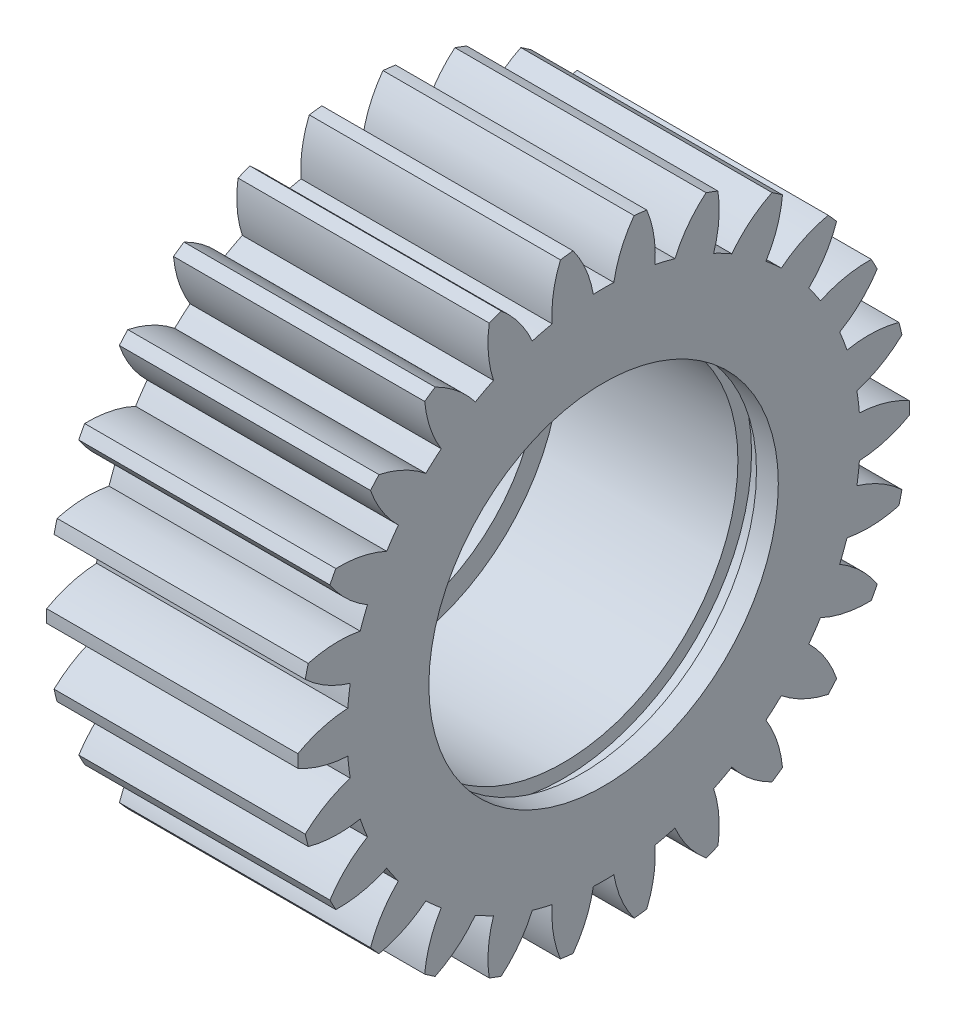
SolidWorks part; units mm, degrees
ref_plane "前视基准面" through (0, 0, 0) normal (0, 0, 1) x (1, 0, 0)
ref_plane "上视基准面" through (0, 0, 0) normal (0, 1, 0) x (1, 0, 0)
ref_plane "右视基准面" through (0, 0, 0) normal (1, 0, 0) x (0, 0, -1)
ref_plane "基准面4" through (0, 0, 0) normal (0, 0, -1) x (-1, 0, 0)
sketch "草图1" plane through (0, 0, 0) normal (0, 0, -1) x (-1, 0, 0)
  line L0 (-20, 28) -> (-20, 0)
  line L1 (-20, 0) -> (3, 0)
  line L2 (3, 0) -> (3, 28)
  line L3 (3, 28) -> (-20, 28)
  line L4 (-20, 0) -> (3, 0) construction
revolve "旋转1" add sketch "草图1" angle 360 about L4
sketch "草图2" plane through (-3, 0, 0) normal (-1, 0, 0) x (0, 0, 1)
  arc A0 (27.0412, 7.2647) -> (25.058, 12.4939) centre (0, 0) ccw
  arc A1 (25.058, 12.4939) -> (21.6211, 9.205) centre (16.3397, 18.1642) cw
  arc A2 (21.6211, 9.205) -> (22.2876, 7.4474) centre (0, 0) cw
  arc A3 (22.2876, 7.4474) -> (27.0412, 7.2647) centre (24.2755, -2.7608) cw
extrude "切除-拉伸1" cut sketch "草图2" against normal through all
sketch "草图3" plane through (-3, 0, 0) normal (-1, 0, 0) x (0, 0, 1)
  arc A0 (27.9939, 0.5822) -> (27.3198, 6.1341) centre (0, 0) ccw
  arc A1 (27.3198, 6.1341) -> (23.1957, 3.7632) centre (20.2119, 13.726) cw
  arc A2 (23.1957, 3.7632) -> (23.4223, 1.8972) centre (0, 0) cw
  arc A3 (23.4223, 1.8972) -> (27.9939, 0.5822) centre (22.9094, -8.4901) cw
extrude "切除-拉伸2" cut sketch "草图3" against normal through all
sketch "草图4" plane through (-3, 0, 0) normal (-1, 0, 0) x (0, 0, 1)
  arc A0 (27.3198, -6.1341) -> (27.9939, -0.5822) centre (0, 0) ccw
  arc A1 (27.9939, -0.5822) -> (23.4223, -1.8972) centre (22.9094, 8.4901) cw
  arc A2 (23.4223, -1.8972) -> (23.1957, -3.7632) centre (0, 0) cw
  arc A3 (23.1957, -3.7632) -> (27.3198, -6.1341) centre (20.2119, -13.726) cw
extrude "切除-拉伸3" cut sketch "草图4" against normal through all
sketch "草图5" plane through (-3, 0, 0) normal (-1, 0, 0) x (0, 0, 1)
  arc A0 (25.058, -12.4939) -> (27.0412, -7.2647) centre (0, 0) ccw
  arc A1 (27.0412, -7.2647) -> (22.2876, -7.4474) centre (24.2755, 2.7608) cw
  arc A2 (22.2876, -7.4474) -> (21.6211, -9.205) centre (0, 0) cw
  arc A3 (21.6211, -9.205) -> (25.058, -12.4939) centre (16.3397, -18.1642) cw
extrude "切除-拉伸4" cut sketch "草图5" against normal through all
sketch "草图6" plane through (-3, 0, 0) normal (-1, 0, 0) x (0, 0, 1)
  arc A0 (21.3399, -18.1276) -> (24.5168, -13.525) centre (0, 0) ccw
  arc A1 (24.5168, -13.525) -> (19.8577, -12.5648) centre (24.2308, -3.1289) cw
  arc A2 (19.8577, -12.5648) -> (18.7899, -14.1118) centre (0, 0) cw
  arc A3 (18.7899, -14.1118) -> (21.3399, -18.1276) centre (11.5179, -21.5467) cw
extrude "切除-拉伸5" cut sketch "草图6" against normal through all
sketch "草图7" plane through (-3, 0, 0) normal (-1, 0, 0) x (0, 0, 1)
  arc A0 (16.3815, -22.7078) -> (20.5677, -18.9992) centre (0, 0) ccw
  arc A1 (20.5677, -18.9992) -> (16.2737, -16.9519) centre (22.7779, -8.8368) cw
  arc A2 (16.2737, -16.9519) -> (14.8668, -18.1984) centre (0, 0) cw
  arc A3 (14.8668, -18.1984) -> (16.3815, -22.7078) centre (6.0268, -23.677) cw
extrude "切除-拉伸6" cut sketch "草图7" against normal through all
sketch "草图8" plane through (-3, 0, 0) normal (-1, 0, 0) x (0, 0, 1)
  arc A0 (15.4232, -23.3693) -> (11.744, -20.3539) centre (20.0013, -14.0311) cw
  arc A1 (11.744, -20.3539) -> (10.0796, -21.2275) centre (0, 0) cw
  arc A2 (10.0796, -21.2275) -> (10.4712, -25.9683) centre (0.1854, -24.4313) cw
  arc A3 (10.4712, -25.9683) -> (15.4232, -23.3693) centre (0, 0) ccw
extrude "切除-拉伸7" cut sketch "草图8" against normal through all
sketch "草图9" plane through (-3, 0, 0) normal (-1, 0, 0) x (0, 0, 1)
  arc A0 (9.3824, -26.3813) -> (6.5317, -22.573) centre (16.0622, -18.41) cw
  arc A1 (6.5317, -22.573) -> (4.7066, -23.0228) centre (0, 0) cw
  arc A2 (4.7066, -23.0228) -> (3.9523, -27.7197) centre (-5.6668, -23.7657) cw
  arc A3 (3.9523, -27.7197) -> (9.3824, -26.3813) centre (0, 0) ccw
extrude "切除-拉伸8" cut sketch "草图9" against normal through all
sketch "草图10" plane through (-3, 0, 0) normal (-1, 0, 0) x (0, 0, 1)
  arc A0 (-2.7963, -27.86) -> (2.7963, -27.86) centre (0, 0) ccw
  arc A1 (2.7963, -27.86) -> (0.9399, -23.4802) centre (11.1896, -21.719) cw
  arc A2 (0.9399, -23.4802) -> (-0.9399, -23.4802) centre (0, 0) cw
  arc A3 (-0.9399, -23.4802) -> (-2.7963, -27.86) centre (-11.1896, -21.719) cw
extrude "切除-拉伸9" cut sketch "草图10" against normal through all
sketch "草图11" plane through (-3, 0, 0) normal (-1, 0, 0) x (0, 0, 1)
  arc A0 (-9.3824, -26.3813) -> (-3.9523, -27.7197) centre (0, 0) ccw
  arc A1 (-3.9523, -27.7197) -> (-4.7066, -23.0228) centre (5.6668, -23.7657) cw
  arc A2 (-4.7066, -23.0228) -> (-6.5317, -22.573) centre (0, 0) cw
  arc A3 (-6.5317, -22.573) -> (-9.3824, -26.3813) centre (-16.0622, -18.41) cw
extrude "切除-拉伸10" cut sketch "草图11" against normal through all
sketch "草图12" plane through (-3, 0, 0) normal (-1, 0, 0) x (0, 0, 1)
  arc A0 (-15.4232, -23.3693) -> (-10.4712, -25.9683) centre (0, 0) ccw
  arc A1 (-10.4712, -25.9683) -> (-10.0796, -21.2275) centre (-0.1854, -24.4313) cw
  arc A2 (-10.0796, -21.2275) -> (-11.744, -20.3539) centre (0, 0) cw
  arc A3 (-11.744, -20.3539) -> (-15.4232, -23.3693) centre (-20.0013, -14.0311) cw
extrude "切除-拉伸11" cut sketch "草图12" against normal through all
sketch "草图13" plane through (-3, 0, 0) normal (-1, 0, 0) x (0, 0, 1)
  arc A0 (-20.5677, -18.9992) -> (-16.3815, -22.7078) centre (0, 0) ccw
  arc A1 (-16.3815, -22.7078) -> (-14.8668, -18.1984) centre (-6.0268, -23.677) cw
  arc A2 (-14.8668, -18.1984) -> (-16.2737, -16.9519) centre (0, 0) cw
  arc A3 (-16.2737, -16.9519) -> (-20.5677, -18.9992) centre (-22.7779, -8.8368) cw
extrude "切除-拉伸12" cut sketch "草图13" against normal through all
sketch "草图14" plane through (-3, 0, 0) normal (-1, 0, 0) x (0, 0, 1)
  arc A0 (-24.5168, -13.525) -> (-21.3399, -18.1276) centre (0, 0) ccw
  arc A1 (-21.3399, -18.1276) -> (-18.7899, -14.1118) centre (-11.5179, -21.5467) cw
  arc A2 (-18.7899, -14.1118) -> (-19.8577, -12.5648) centre (0, 0) cw
  arc A3 (-19.8577, -12.5648) -> (-24.5168, -13.525) centre (-24.2308, -3.1289) cw
extrude "切除-拉伸13" cut sketch "草图14" against normal through all
sketch "草图15" plane through (-3, 0, 0) normal (-1, 0, 0) x (0, 0, 1)
  arc A0 (-27.0412, -7.2647) -> (-25.058, -12.4939) centre (0, 0) ccw
  arc A1 (-25.058, -12.4939) -> (-21.6211, -9.205) centre (-16.3397, -18.1642) cw
  arc A2 (-21.6211, -9.205) -> (-22.2876, -7.4474) centre (0, 0) cw
  arc A3 (-22.2876, -7.4474) -> (-27.0412, -7.2647) centre (-24.2755, 2.7608) cw
extrude "切除-拉伸14" cut sketch "草图15" against normal through all
sketch "草图16" plane through (-3, 0, 0) normal (-1, 0, 0) x (0, 0, 1)
  arc A0 (-27.9939, -0.5822) -> (-27.3198, -6.1341) centre (0, 0) ccw
  arc A1 (-27.3198, -6.1341) -> (-23.1957, -3.7632) centre (-20.2119, -13.726) cw
  arc A2 (-23.1957, -3.7632) -> (-23.4223, -1.8972) centre (0, 0) cw
  arc A3 (-23.4223, -1.8972) -> (-27.9939, -0.5822) centre (-22.9094, 8.4901) cw
extrude "切除-拉伸15" cut sketch "草图16" against normal through all
sketch "草图17" plane through (-3, 0, 0) normal (-1, 0, 0) x (0, 0, 1)
  arc A0 (-27.3198, 6.1341) -> (-27.9939, 0.5822) centre (0, 0) ccw
  arc A1 (-27.9939, 0.5822) -> (-23.4223, 1.8972) centre (-22.9094, -8.4901) cw
  arc A2 (-23.4223, 1.8972) -> (-23.1957, 3.7632) centre (0, 0) cw
  arc A3 (-23.1957, 3.7632) -> (-27.3198, 6.1341) centre (-20.2119, 13.726) cw
extrude "切除-拉伸16" cut sketch "草图17" against normal through all
sketch "草图18" plane through (-3, 0, 0) normal (-1, 0, 0) x (0, 0, 1)
  arc A0 (-25.058, 12.4939) -> (-27.0412, 7.2647) centre (0, 0) ccw
  arc A1 (-27.0412, 7.2647) -> (-22.2876, 7.4474) centre (-24.2755, -2.7608) cw
  arc A2 (-22.2876, 7.4474) -> (-21.6211, 9.205) centre (0, 0) cw
  arc A3 (-21.6211, 9.205) -> (-25.058, 12.4939) centre (-16.3397, 18.1642) cw
extrude "切除-拉伸17" cut sketch "草图18" against normal through all
sketch "草图19" plane through (-3, 0, 0) normal (-1, 0, 0) x (0, 0, 1)
  arc A0 (-21.3399, 18.1276) -> (-24.5168, 13.525) centre (0, 0) ccw
  arc A1 (-24.5168, 13.525) -> (-19.8577, 12.5648) centre (-24.2308, 3.1289) cw
  arc A2 (-19.8577, 12.5648) -> (-18.7899, 14.1118) centre (0, 0) cw
  arc A3 (-18.7899, 14.1118) -> (-21.3399, 18.1276) centre (-11.5179, 21.5467) cw
extrude "切除-拉伸18" cut sketch "草图19" against normal through all
sketch "草图20" plane through (-3, 0, 0) normal (-1, 0, 0) x (0, 0, 1)
  arc A0 (-16.3815, 22.7078) -> (-20.5677, 18.9992) centre (0, 0) ccw
  arc A1 (-20.5677, 18.9992) -> (-16.2737, 16.9519) centre (-22.7779, 8.8368) cw
  arc A2 (-16.2737, 16.9519) -> (-14.8668, 18.1984) centre (0, 0) cw
  arc A3 (-14.8668, 18.1984) -> (-16.3815, 22.7078) centre (-6.0268, 23.677) cw
extrude "切除-拉伸19" cut sketch "草图20" against normal through all
sketch "草图21" plane through (-3, 0, 0) normal (-1, 0, 0) x (0, 0, 1)
  arc A0 (-10.4712, 25.9683) -> (-15.4232, 23.3693) centre (0, 0) ccw
  arc A1 (-15.4232, 23.3693) -> (-11.744, 20.3539) centre (-20.0013, 14.0311) cw
  arc A2 (-11.744, 20.3539) -> (-10.0796, 21.2275) centre (0, 0) cw
  arc A3 (-10.0796, 21.2275) -> (-10.4712, 25.9683) centre (-0.1854, 24.4313) cw
extrude "切除-拉伸20" cut sketch "草图21" against normal through all
sketch "草图22" plane through (-3, 0, 0) normal (-1, 0, 0) x (0, 0, 1)
  arc A0 (-3.9523, 27.7197) -> (-9.3824, 26.3813) centre (0, 0) ccw
  arc A1 (-9.3824, 26.3813) -> (-6.5317, 22.573) centre (-16.0622, 18.41) cw
  arc A2 (-6.5317, 22.573) -> (-4.7066, 23.0228) centre (0, 0) cw
  arc A3 (-4.7066, 23.0228) -> (-3.9523, 27.7197) centre (5.6668, 23.7657) cw
extrude "切除-拉伸21" cut sketch "草图22" against normal through all
sketch "草图23" plane through (-3, 0, 0) normal (-1, 0, 0) x (0, 0, 1)
  arc A0 (2.7963, 27.86) -> (-2.7963, 27.86) centre (0, 0) ccw
  arc A1 (-2.7963, 27.86) -> (-0.9399, 23.4802) centre (-11.1896, 21.719) cw
  arc A2 (-0.9399, 23.4802) -> (0.9399, 23.4802) centre (0, 0) cw
  arc A3 (0.9399, 23.4802) -> (2.7963, 27.86) centre (11.1896, 21.719) cw
extrude "切除-拉伸22" cut sketch "草图23" against normal through all
sketch "草图24" plane through (-3, 0, 0) normal (-1, 0, 0) x (0, 0, 1)
  arc A0 (9.3824, 26.3813) -> (3.9523, 27.7197) centre (0, 0) ccw
  arc A1 (3.9523, 27.7197) -> (4.7066, 23.0228) centre (-5.6668, 23.7657) cw
  arc A2 (4.7066, 23.0228) -> (6.5317, 22.573) centre (0, 0) cw
  arc A3 (6.5317, 22.573) -> (9.3824, 26.3813) centre (16.0622, 18.41) cw
extrude "切除-拉伸23" cut sketch "草图24" against normal through all
sketch "草图25" plane through (-3, 0, 0) normal (-1, 0, 0) x (0, 0, 1)
  arc A0 (15.4232, 23.3693) -> (10.4712, 25.9683) centre (0, 0) ccw
  arc A1 (10.4712, 25.9683) -> (10.0796, 21.2275) centre (0.1854, 24.4313) cw
  arc A2 (10.0796, 21.2275) -> (11.744, 20.3539) centre (0, 0) cw
  arc A3 (11.744, 20.3539) -> (15.4232, 23.3693) centre (20.0013, 14.0311) cw
extrude "切除-拉伸24" cut sketch "草图25" against normal through all
sketch "草图26" plane through (-3, 0, 0) normal (-1, 0, 0) x (0, 0, 1)
  arc A0 (20.5677, 18.9992) -> (16.3815, 22.7078) centre (0, 0) ccw
  arc A1 (16.3815, 22.7078) -> (14.8668, 18.1984) centre (6.0268, 23.677) cw
  arc A2 (14.8668, 18.1984) -> (16.2737, 16.9519) centre (0, 0) cw
  arc A3 (16.2737, 16.9519) -> (20.5677, 18.9992) centre (22.7779, 8.8368) cw
extrude "切除-拉伸25" cut sketch "草图26" against normal through all
sketch "草图27" plane through (-3, 0, 0) normal (-1, 0, 0) x (0, 0, 1)
  arc A0 (24.5168, 13.525) -> (21.3399, 18.1276) centre (0, 0) ccw
  arc A1 (21.3399, 18.1276) -> (18.7899, 14.1118) centre (11.5179, 21.5467) cw
  arc A2 (18.7899, 14.1118) -> (19.8577, 12.5648) centre (0, 0) cw
  arc A3 (19.8577, 12.5648) -> (24.5168, 13.525) centre (24.2308, 3.1289) cw
extrude "切除-拉伸26" cut sketch "草图27" against normal through all
sketch "草图28" plane through (0, 0, 0) normal (0, 0, 1) x (1, 0, 0)
  line L0 (-3, 14) -> (-3, 0)
  line L1 (-3, 0) -> (20, 0)
  line L2 (20, 0) -> (20, 16)
  line L3 (20, 16) -> (18, 16)
  line L4 (18, 16) -> (18, 17.25)
  line L5 (18, 17.25) -> (16.3, 17.25)
  line L6 (16.3, 17.25) -> (16.3, 16)
  line L7 (16.3, 16) -> (0, 16)
  line L8 (0, 16) -> (0, 14)
  line L9 (0, 14) -> (-3, 14)
  line L10 (-3, 0) -> (20, 0) construction
revolve "切除-旋转1" cut sketch "草图28" angle 360 about L10
sketch "草图29" plane through (-3, 0, 0) normal (-1, 0, 0) x (0, 0, 1)
  circle A0 centre (0, 0) radius 26 construction
  dimension "D1" = 52
